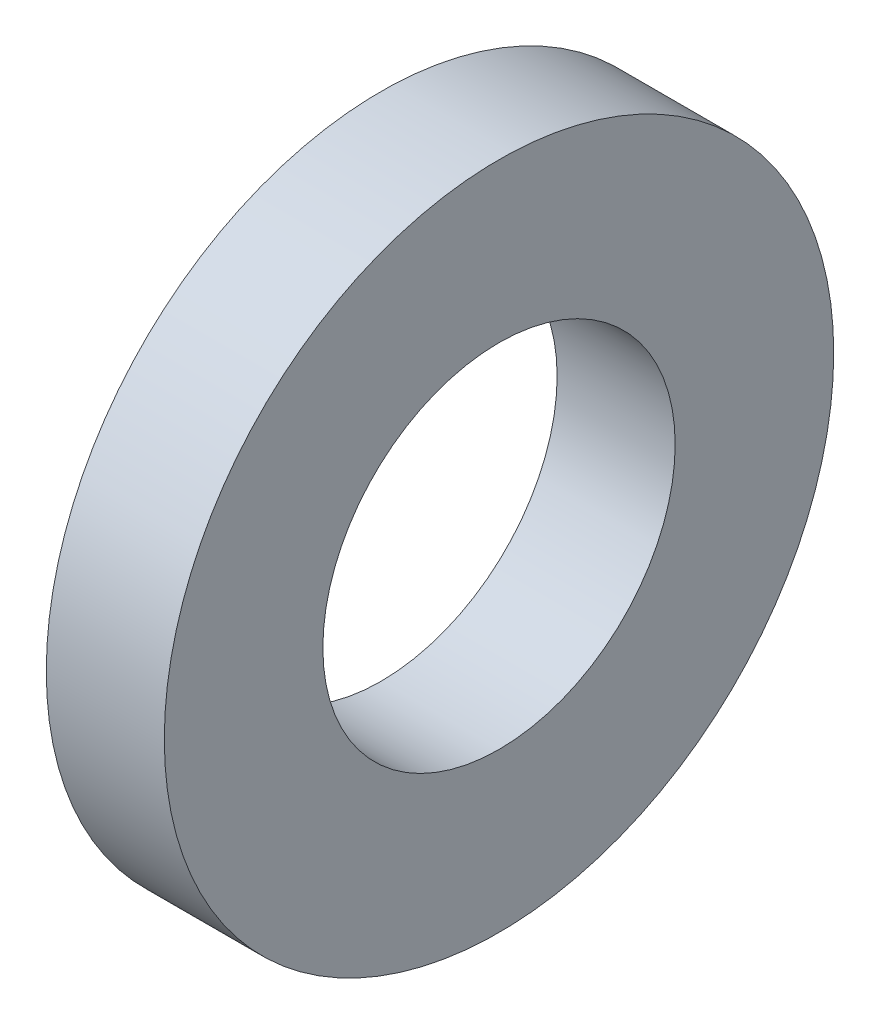
from build123d import *

# Parameters (mm, degrees)
SKETCH1_R           = 19
SKETCH1_R_2         = 10
BOSS_EXTRUDE1_DEPTH = 6.7


with BuildPart() as part:
    # Sketch1 → Boss-Extrude1 (new body)
    with BuildSketch(Plane(origin=(0, 0, 0), x_dir=(0, 0, -1), z_dir=(1, 0, 0))):
        Circle(SKETCH1_R)
        Circle(SKETCH1_R_2, mode=Mode.SUBTRACT)
    extrude(amount=BOSS_EXTRUDE1_DEPTH)


solid = part.part
